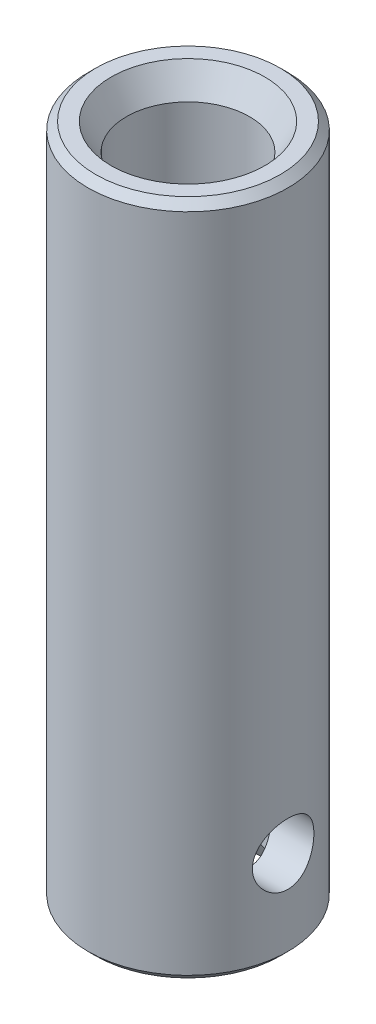
SolidWorks part; units mm, degrees
ref_plane "前视基准面" through (0, 0, 0) normal (0, 0, 1) x (1, 0, 0)
ref_plane "上视基准面" through (0, 0, 0) normal (0, 1, 0) x (1, 0, 0)
ref_plane "右视基准面" through (0, 0, 0) normal (1, 0, 0) x (0, 0, -1)
sketch "草图1" plane through (0, 0, 0) normal (0, 1, 0) x (1, 0, 0)
  circle A0 centre (0, 0) radius 6.5
  circle A1 centre (0, 0) radius 4
  dimension "D1" = 13
  dimension "D2" = 8
extrude "凸台-拉伸1" add sketch "草图1" along normal blind 44
hole_wizard "Ø4.0 (4) 直径孔1" positions "3D草图1" profile "草图2" hole size "Ø4.0" standard "GB" end condition through all
sketch3d "3D草图1"
  point P0 (6.5, 6, 0)
  dimension "D1" = 38
sketch "草图2" plane through (6.5, 6, 0) normal (0, 1, 0) x (0, 0, -1)
  line L0 (0, 0) -> (0, 13)
  line L1 (0, 13) -> (2, 13)
  line L2 (2, 13) -> (2, 0)
  line L5 (2, 0) -> (0, 0)
  line L11 (0, -6.35) -> (0, 107.95) construction
  dimension "通孔孔直径" = 4
  dimension "通孔孔深度" = 13
chamfer "倒角1" distance 0.5 angle 45 2 edges at (0, 0, 6.5) (0, 44, 6.5)
chamfer "倒角2" distance 1 angle 60 2 edges at (0, 0, 4) (0, 44, 4)
